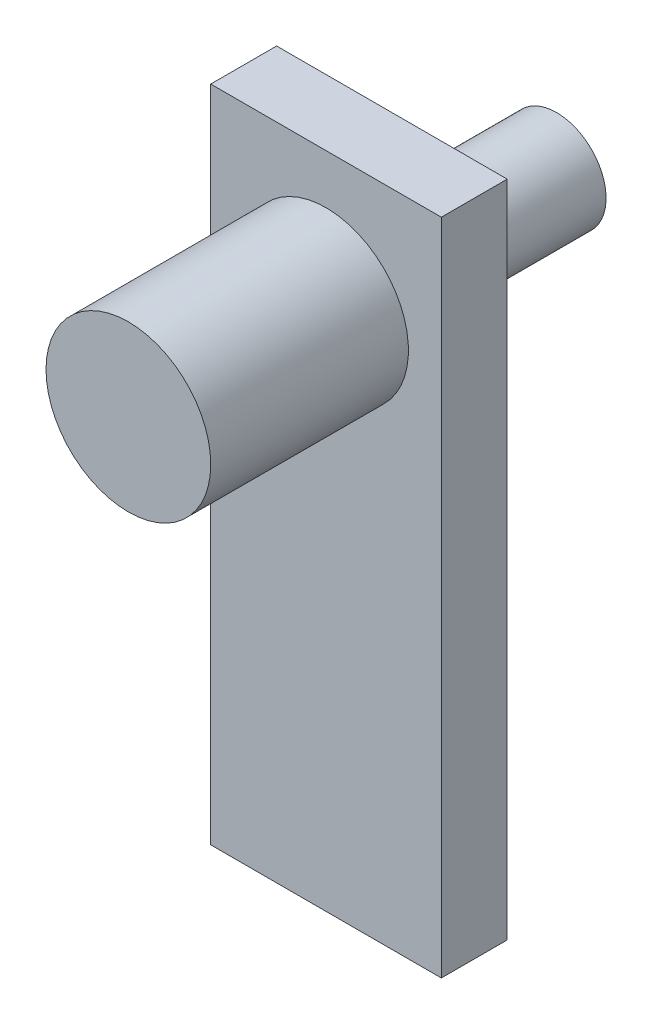
SolidWorks part; units mm, degrees
ref_plane "前视基准面" through (0, 0, 0) normal (0, 0, 1) x (1, 0, 0)
ref_plane "上视基准面" through (0, 0, 0) normal (0, 1, 0) x (1, 0, 0)
ref_plane "右视基准面" through (0, 0, 0) normal (1, 0, 0) x (0, 0, -1)
sketch "草图1" plane through (0, 0, 0) normal (0, 0, 1) x (1, 0, 0)
  line L1 (-17.5, -50) -> (17.5, -50)
  line L2 (-17.5, -50) -> (-17.5, 50)
  line L3 (-17.5, 50) -> (17.5, 50)
  line L4 (17.5, -50) -> (17.5, 50)
  line L5 (-17.5, -50) -> (17.5, 50) construction
  line L6 (-17.5, 50) -> (17.5, -50) construction
  point P0 (0, 0)
  dimension "D1" = 35
  dimension "D2" = 100
extrude "凸台-拉伸1" add sketch "草图1" along normal blind 10
sketch "草图2" plane through (0, 0, 10) normal (0, 0, 1) x (1, 0, 0)
  line L0 (0, 0) -> (0, 50) construction
  line L1 (17.5, 50) -> (-17.5, 50) construction
  circle A0 centre (0, 30) radius 12.5
  dimension "D1" = 25
  dimension "D2" = 20
extrude "凸台-拉伸2" add sketch "草图2" along normal blind 30
sketch "草图3" plane through (0, 0, 0) normal (0, 0, -1) x (-1, 0, 0)
  line L0 (0, 0) -> (0, 50) construction
  line L1 (-17.5, 50) -> (17.5, 50) construction
  circle A0 centre (0, 30) radius 7.5
  dimension "D1" = 15
  dimension "D2" = 20
extrude "凸台-拉伸3" add sketch "草图3" along normal blind 25
